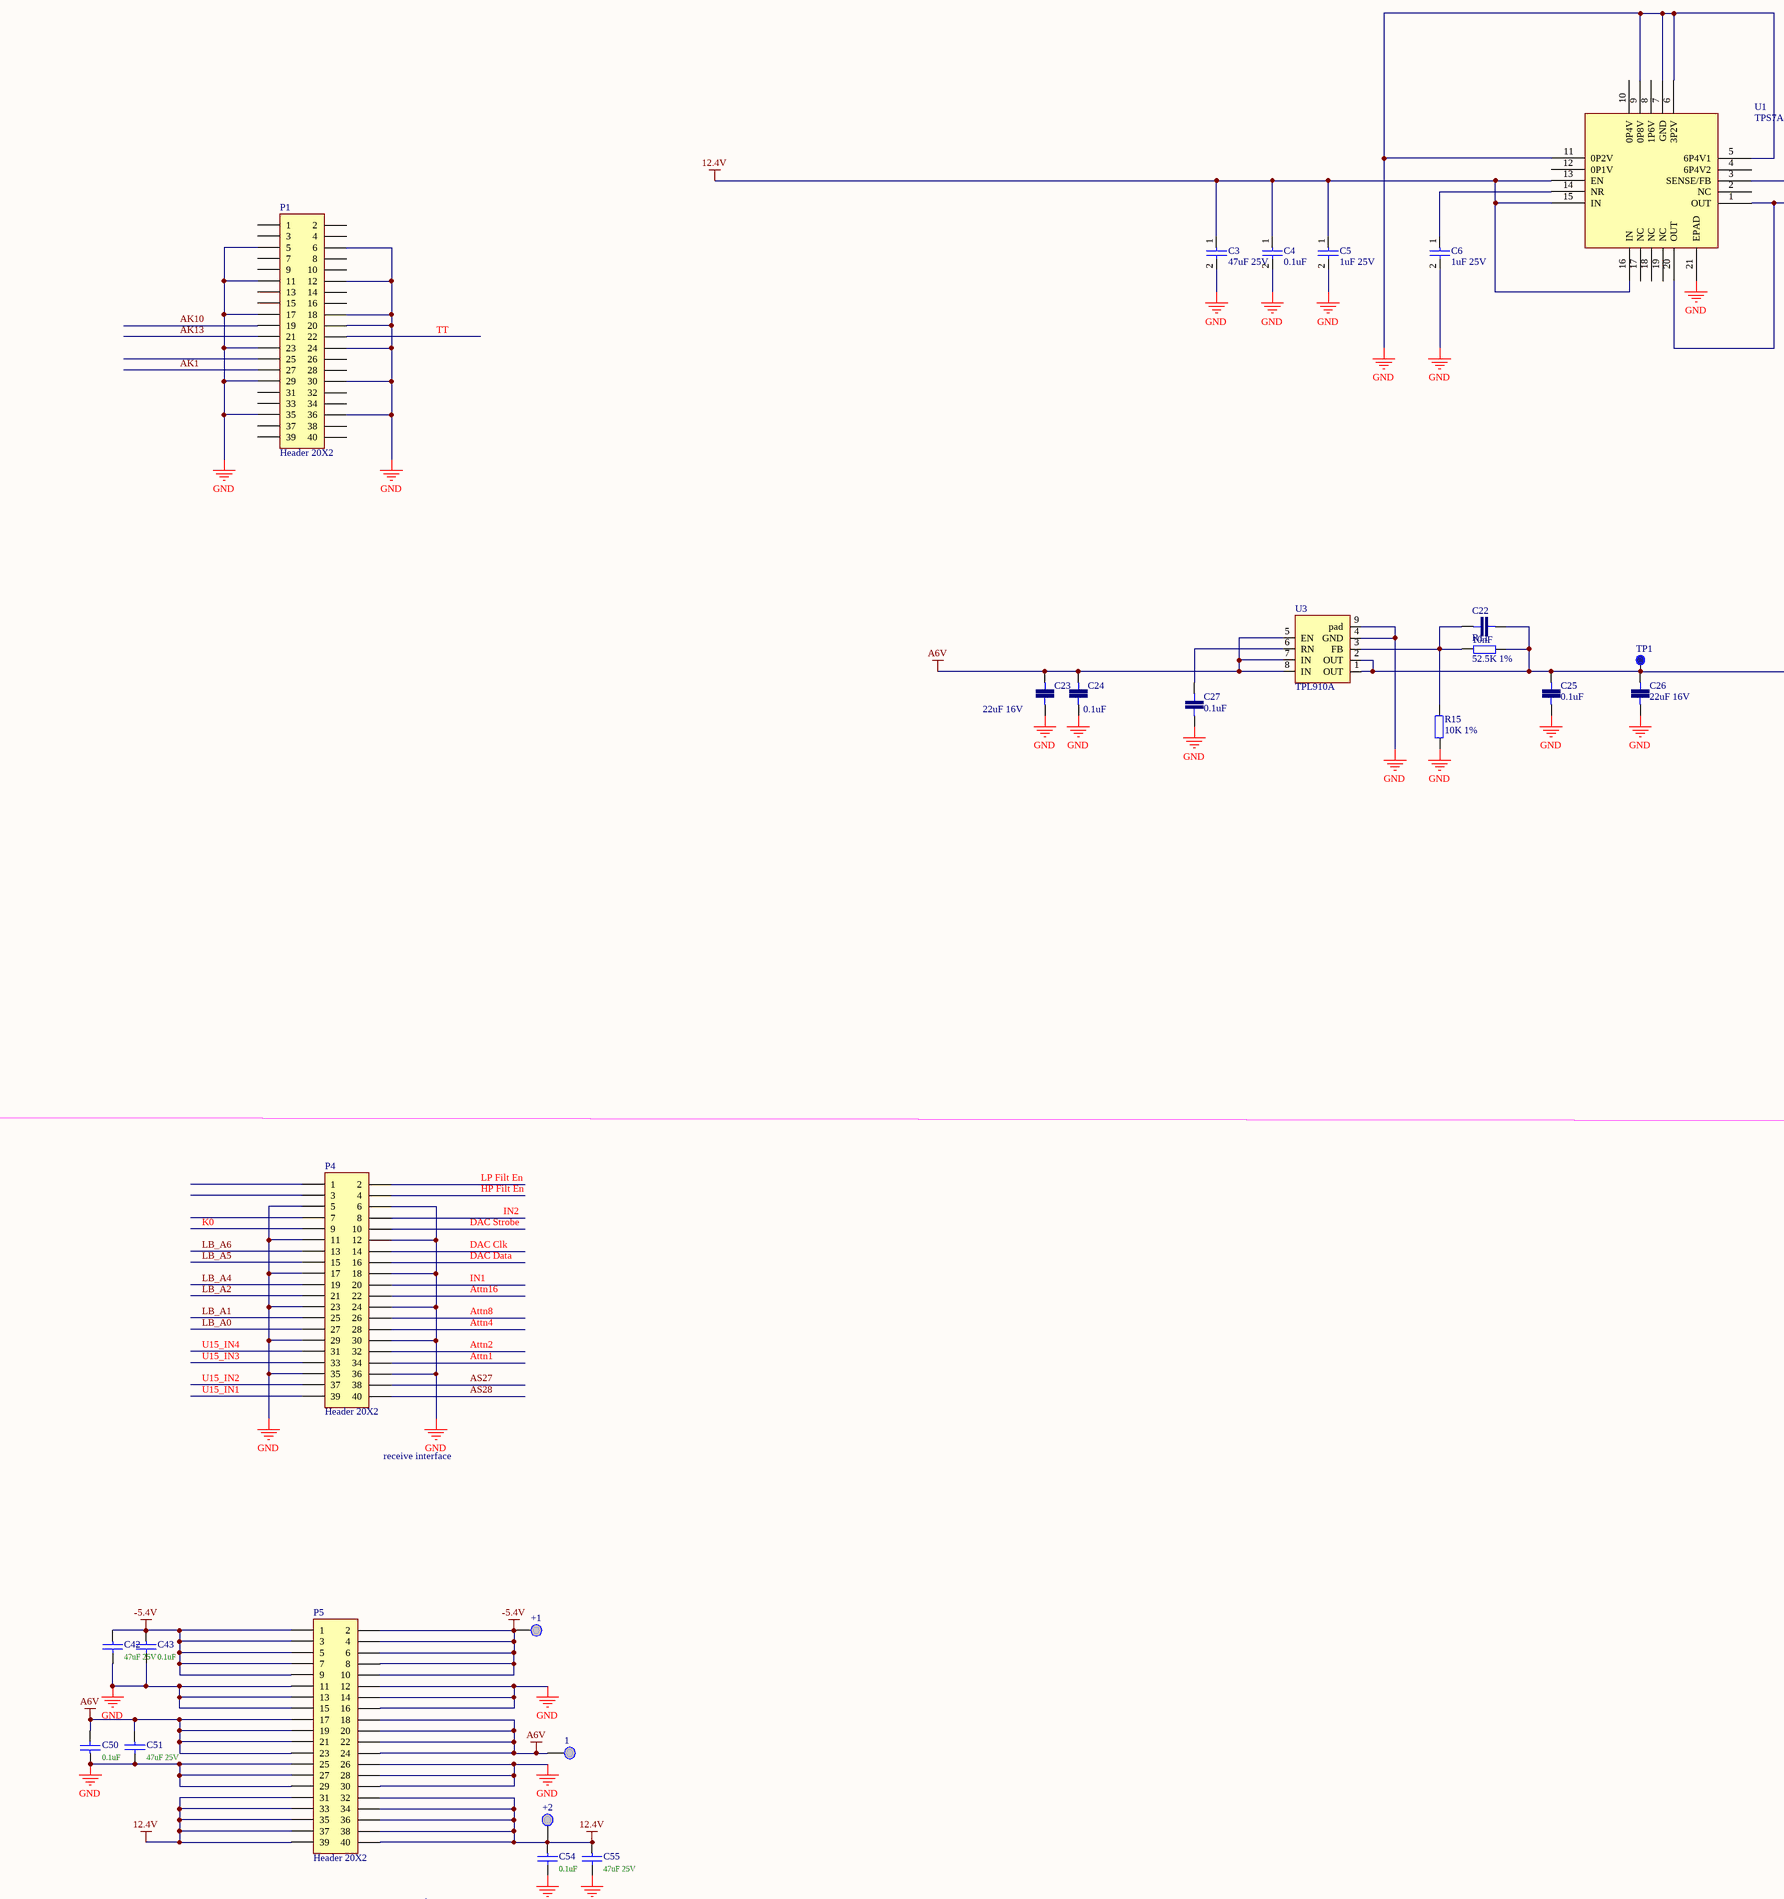
[diagram p0: PCBE109358.SchDoc, top column 1 of 4]
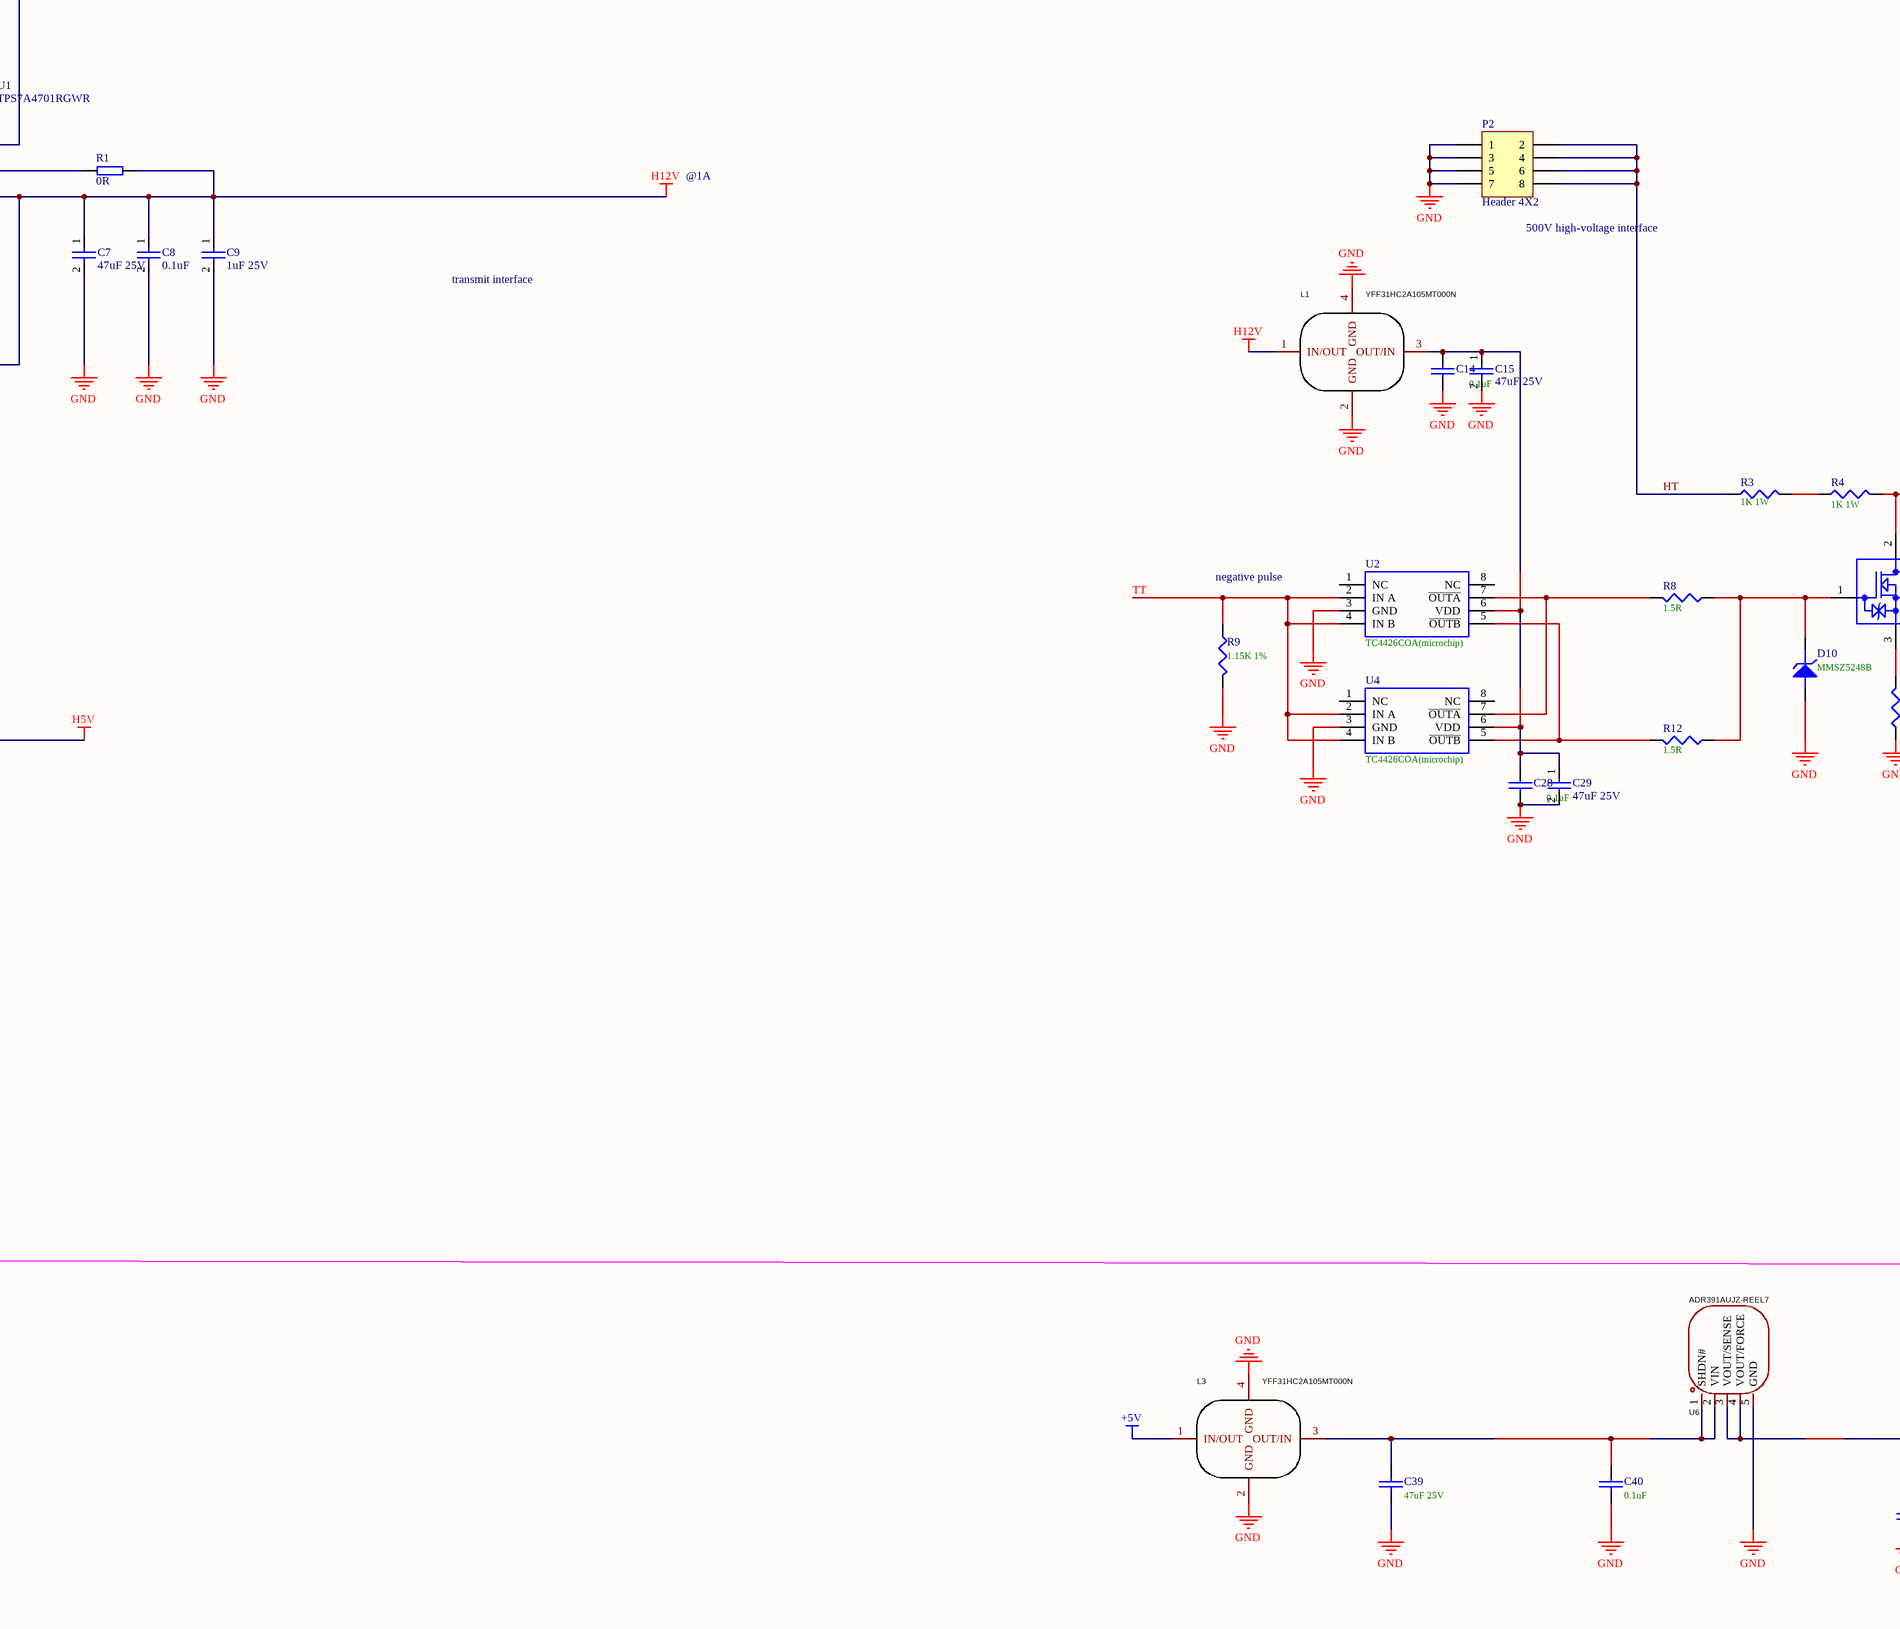
[diagram p1: PCBE109358.SchDoc, top column 2 of 4]
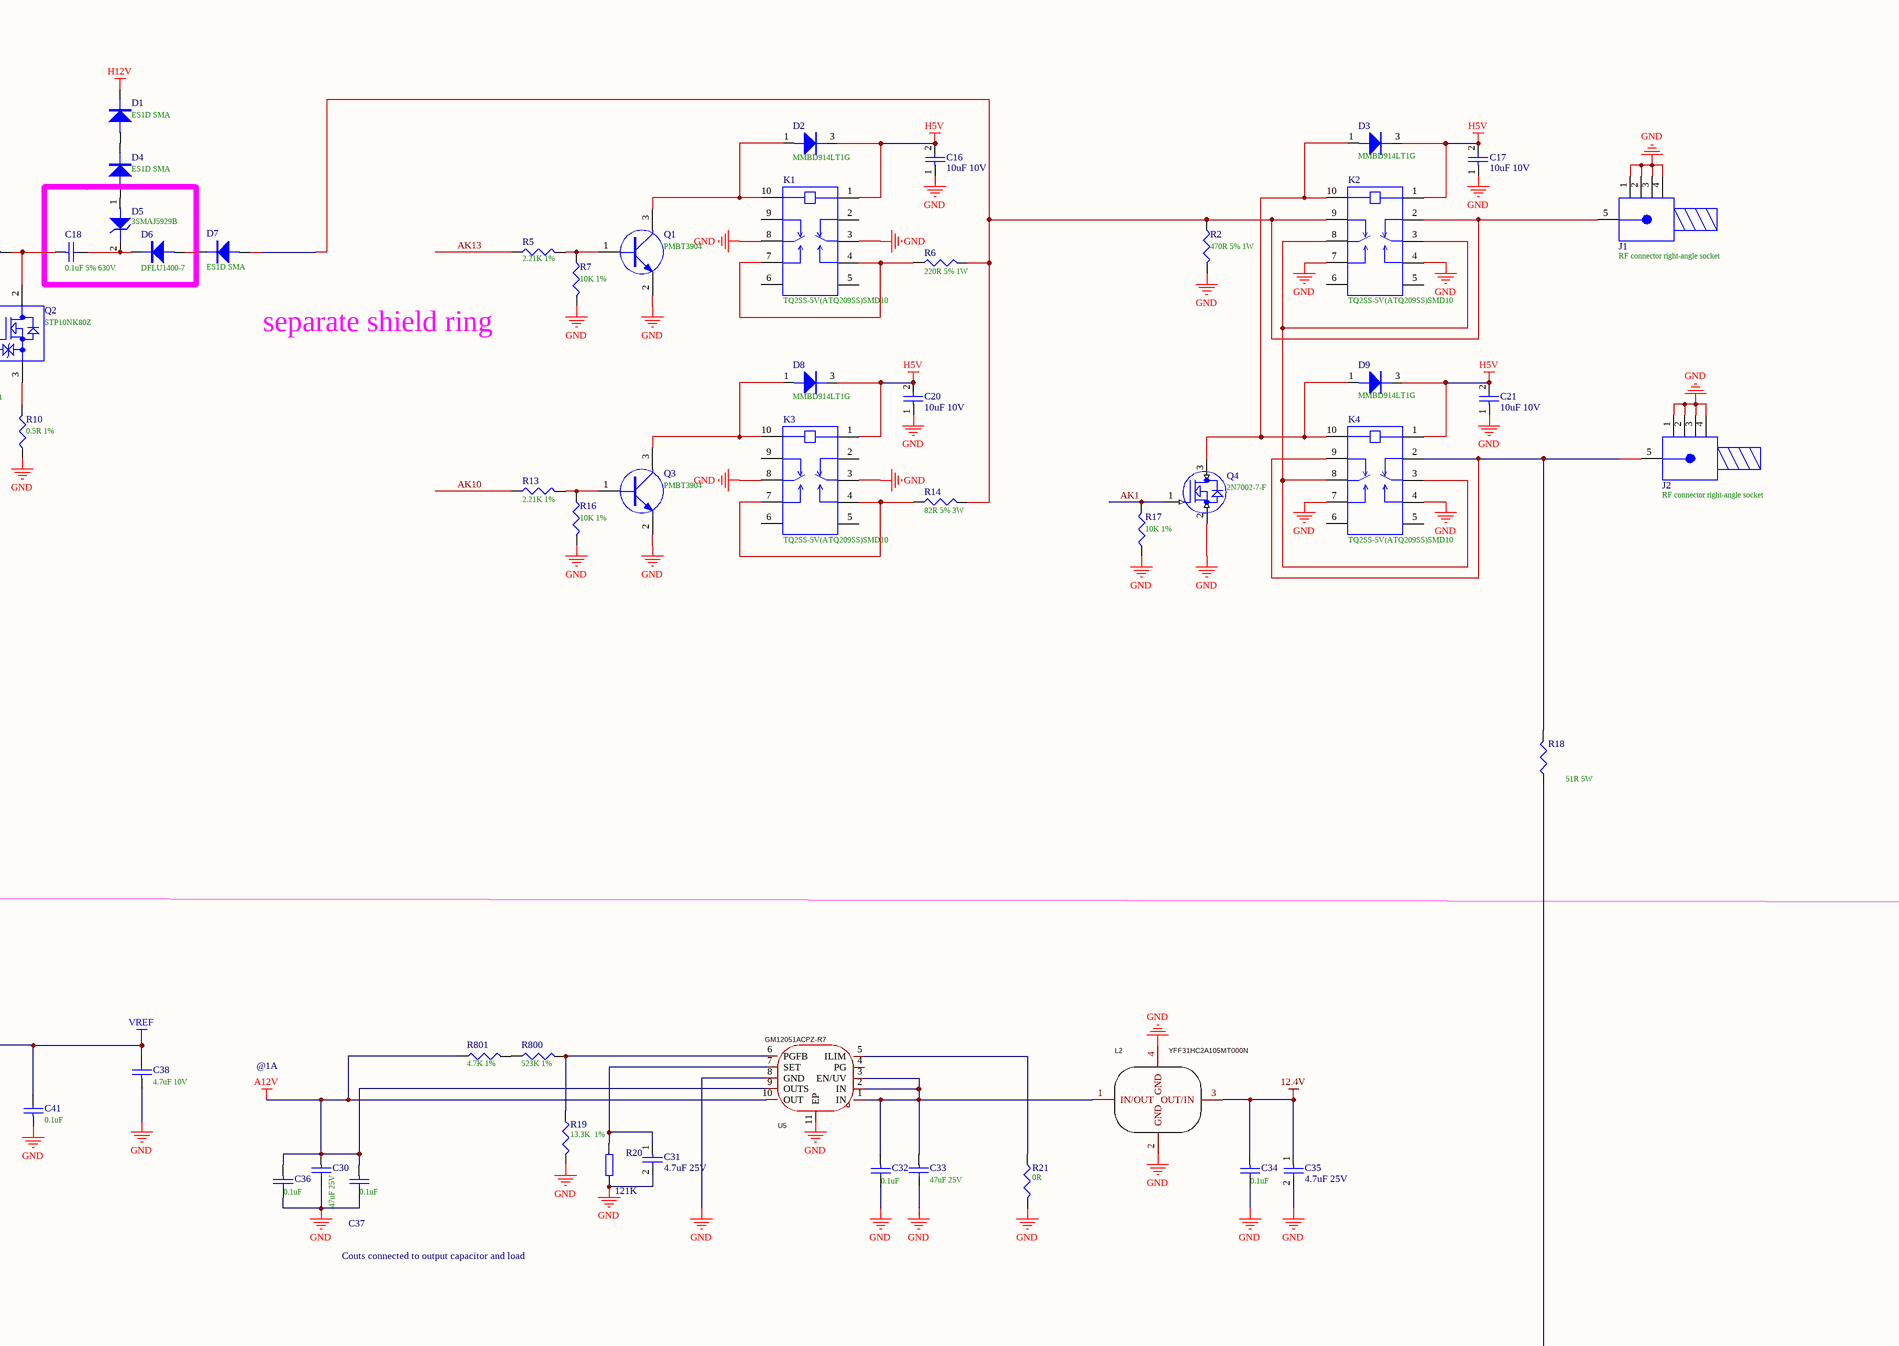
[diagram p2: PCBE109358.SchDoc, top column 3 of 4]
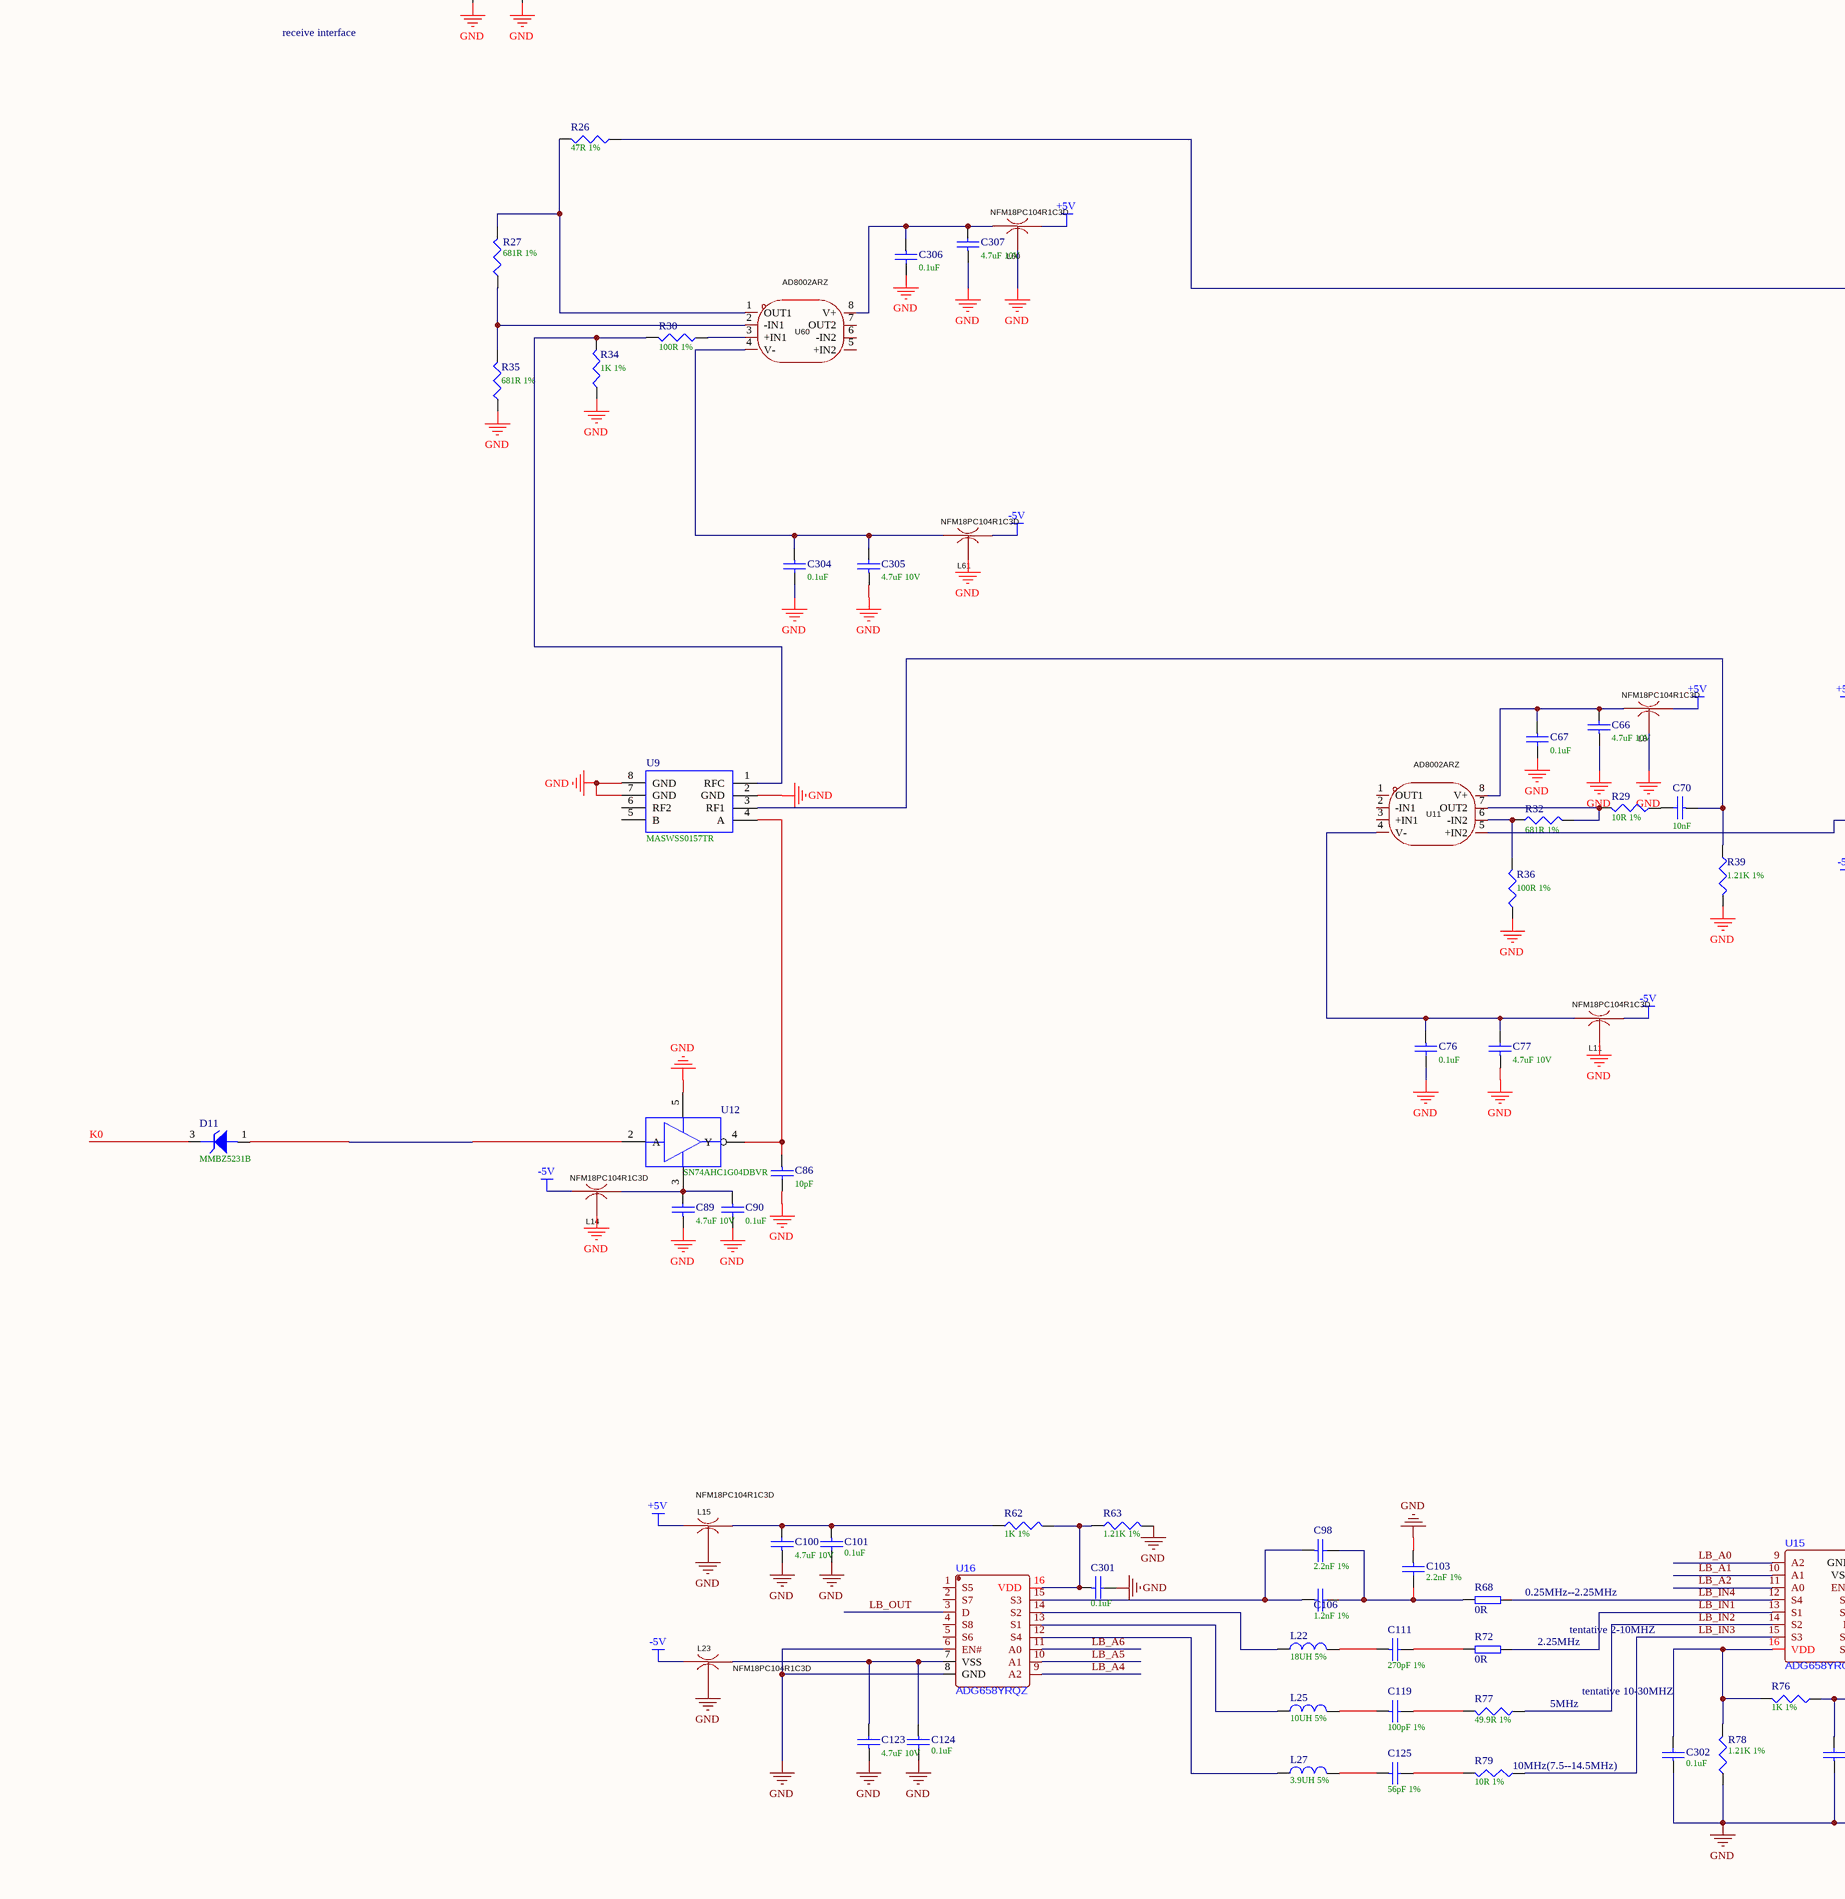
[diagram p3: PCBE109358.SchDoc, bottom column 1 of 4]
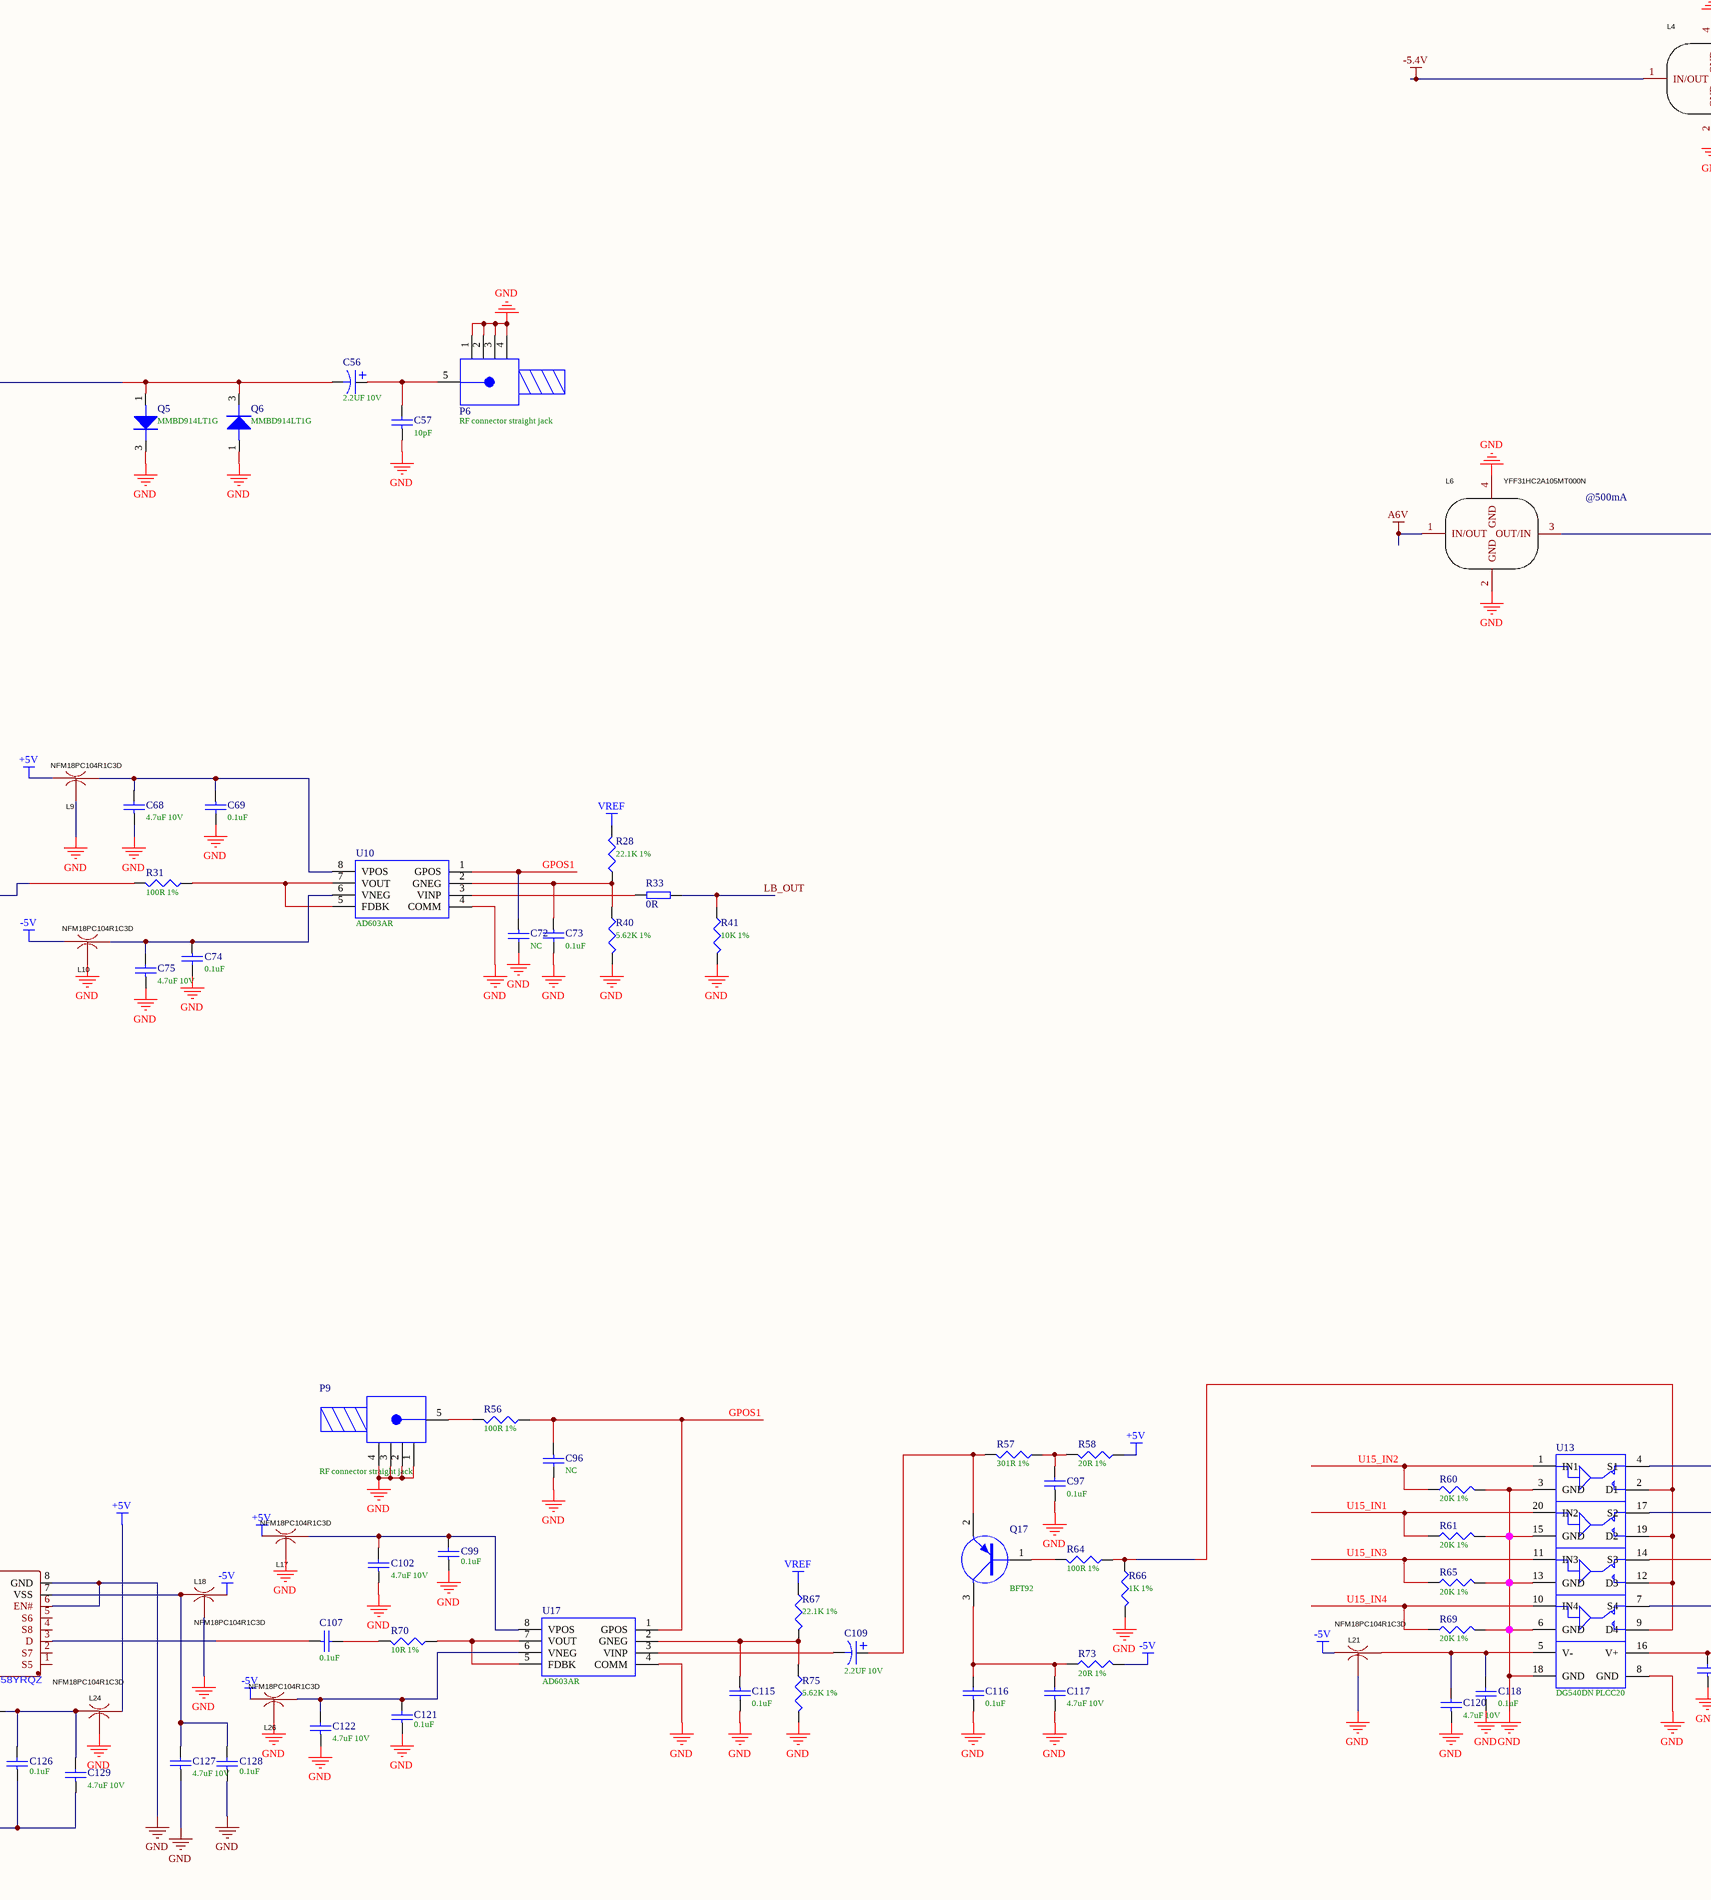
[diagram p4: PCBE109358.SchDoc, bottom column 2 of 4]
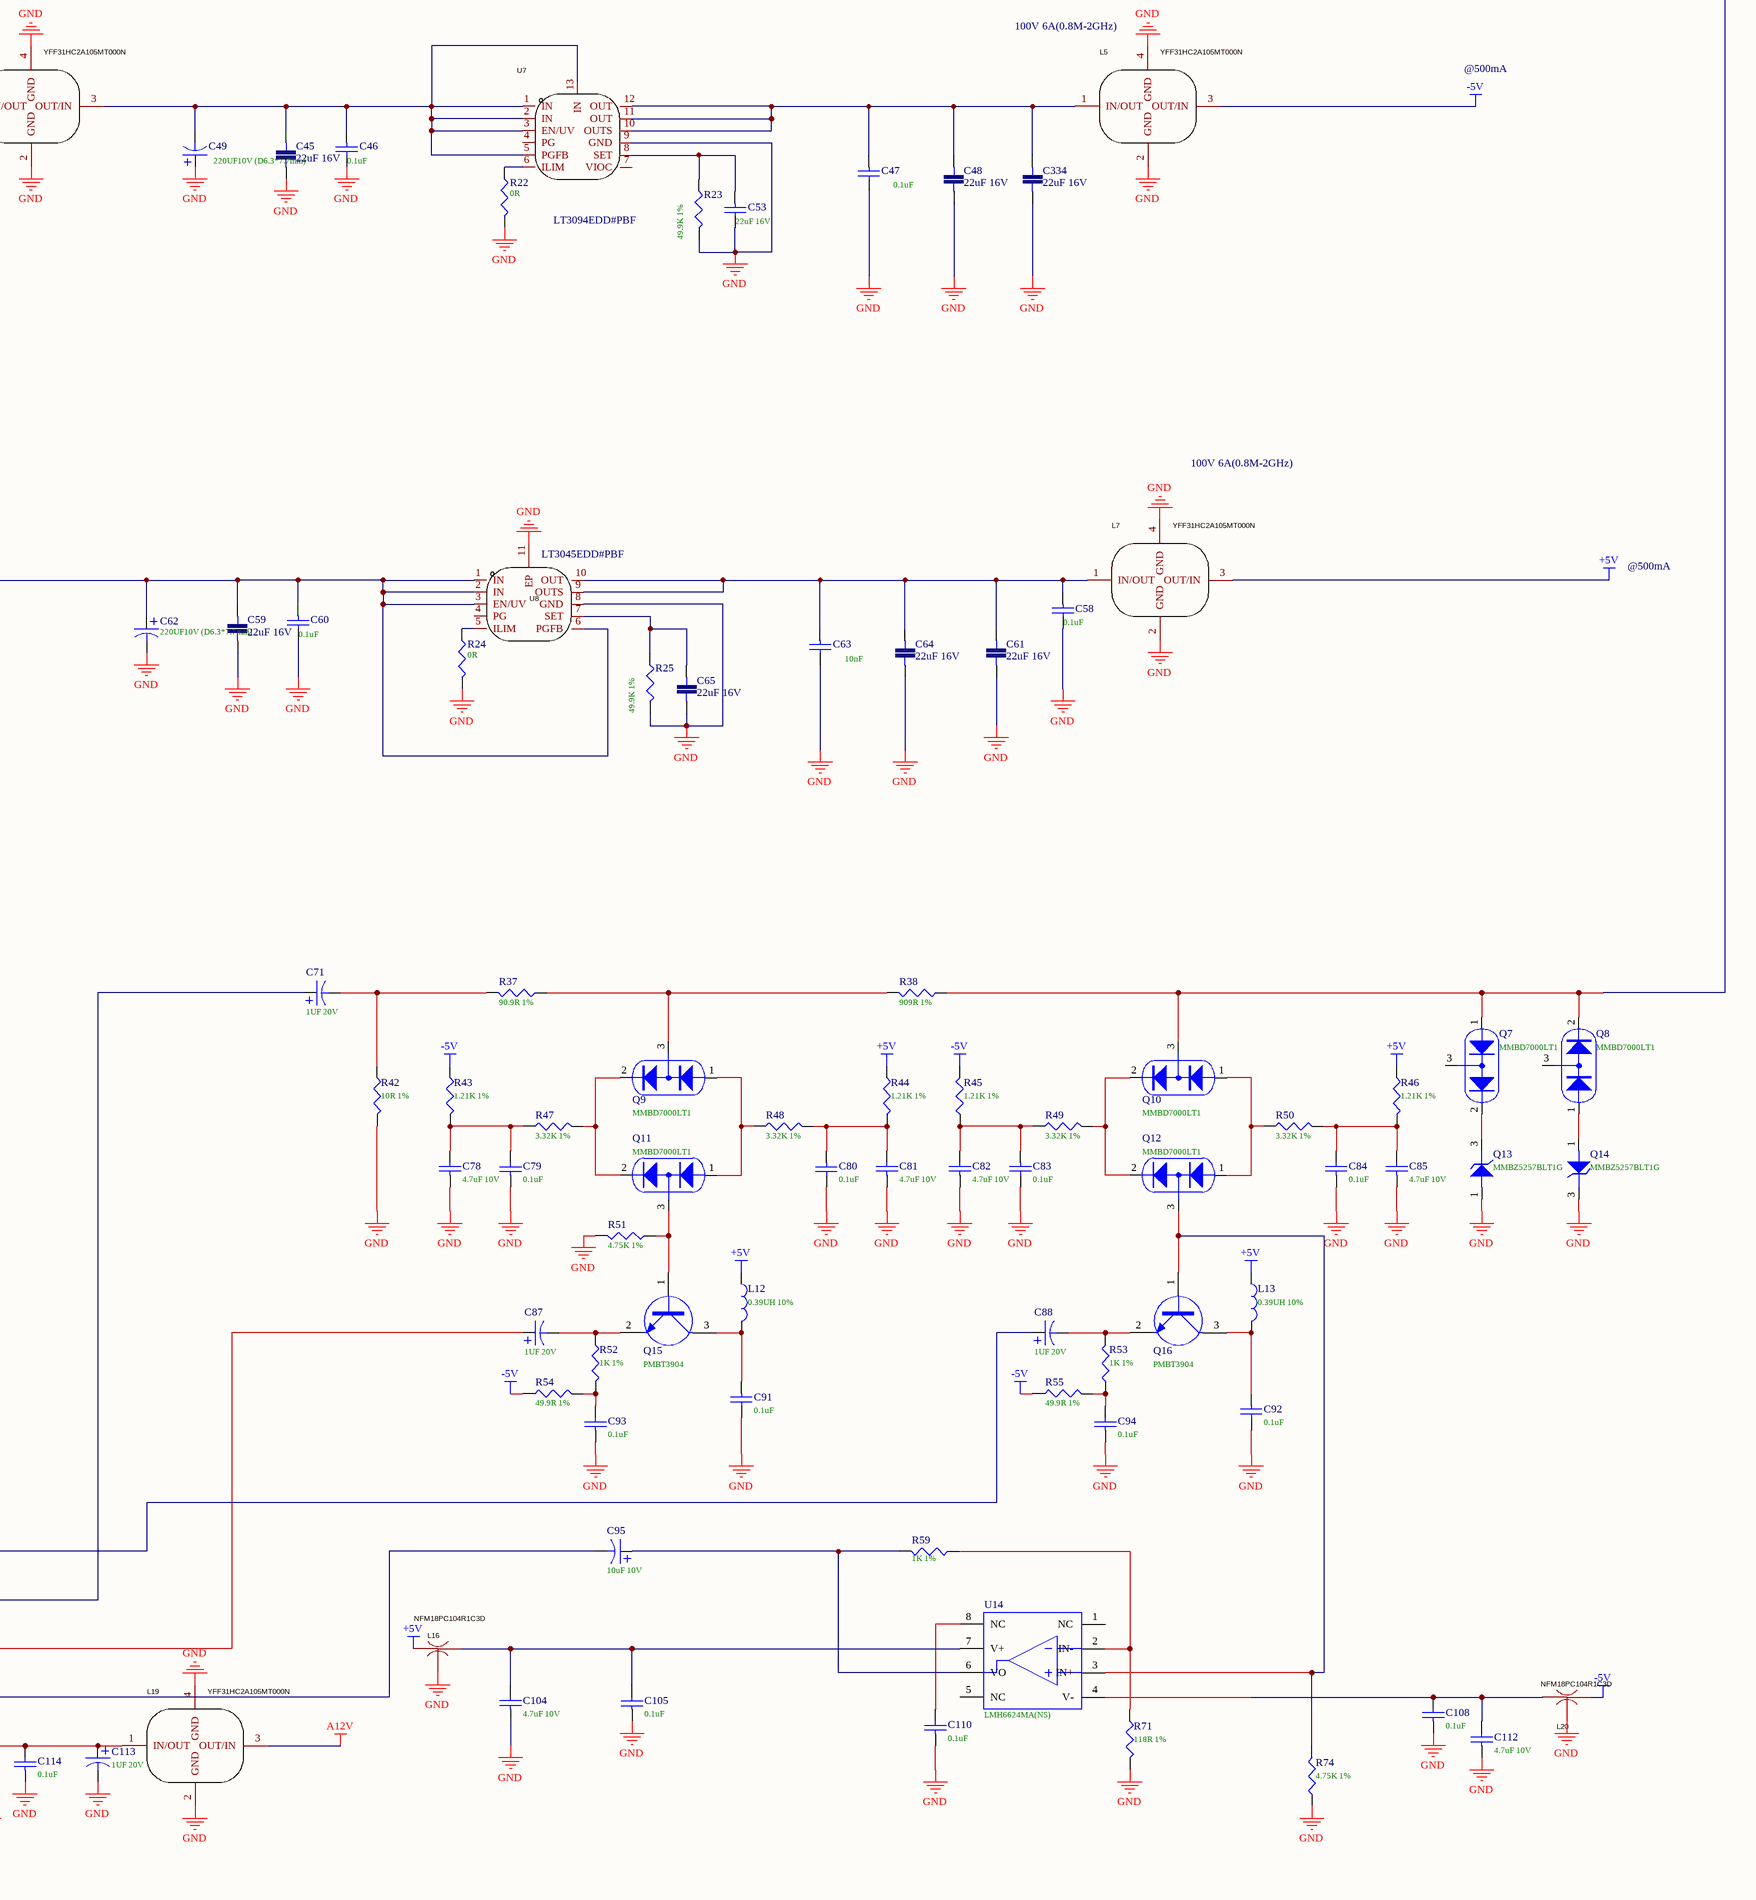
[diagram p5: PCBE109358.SchDoc, bottom column 3 of 4]
# Altium project MISC109358-2.PrjPcb (part 1 of 2)
1 sheet, 299 parts. Net scope: global (net labels, ports and power ports of the same name join across sheets).
Board file: MISC109358.PcbDoc